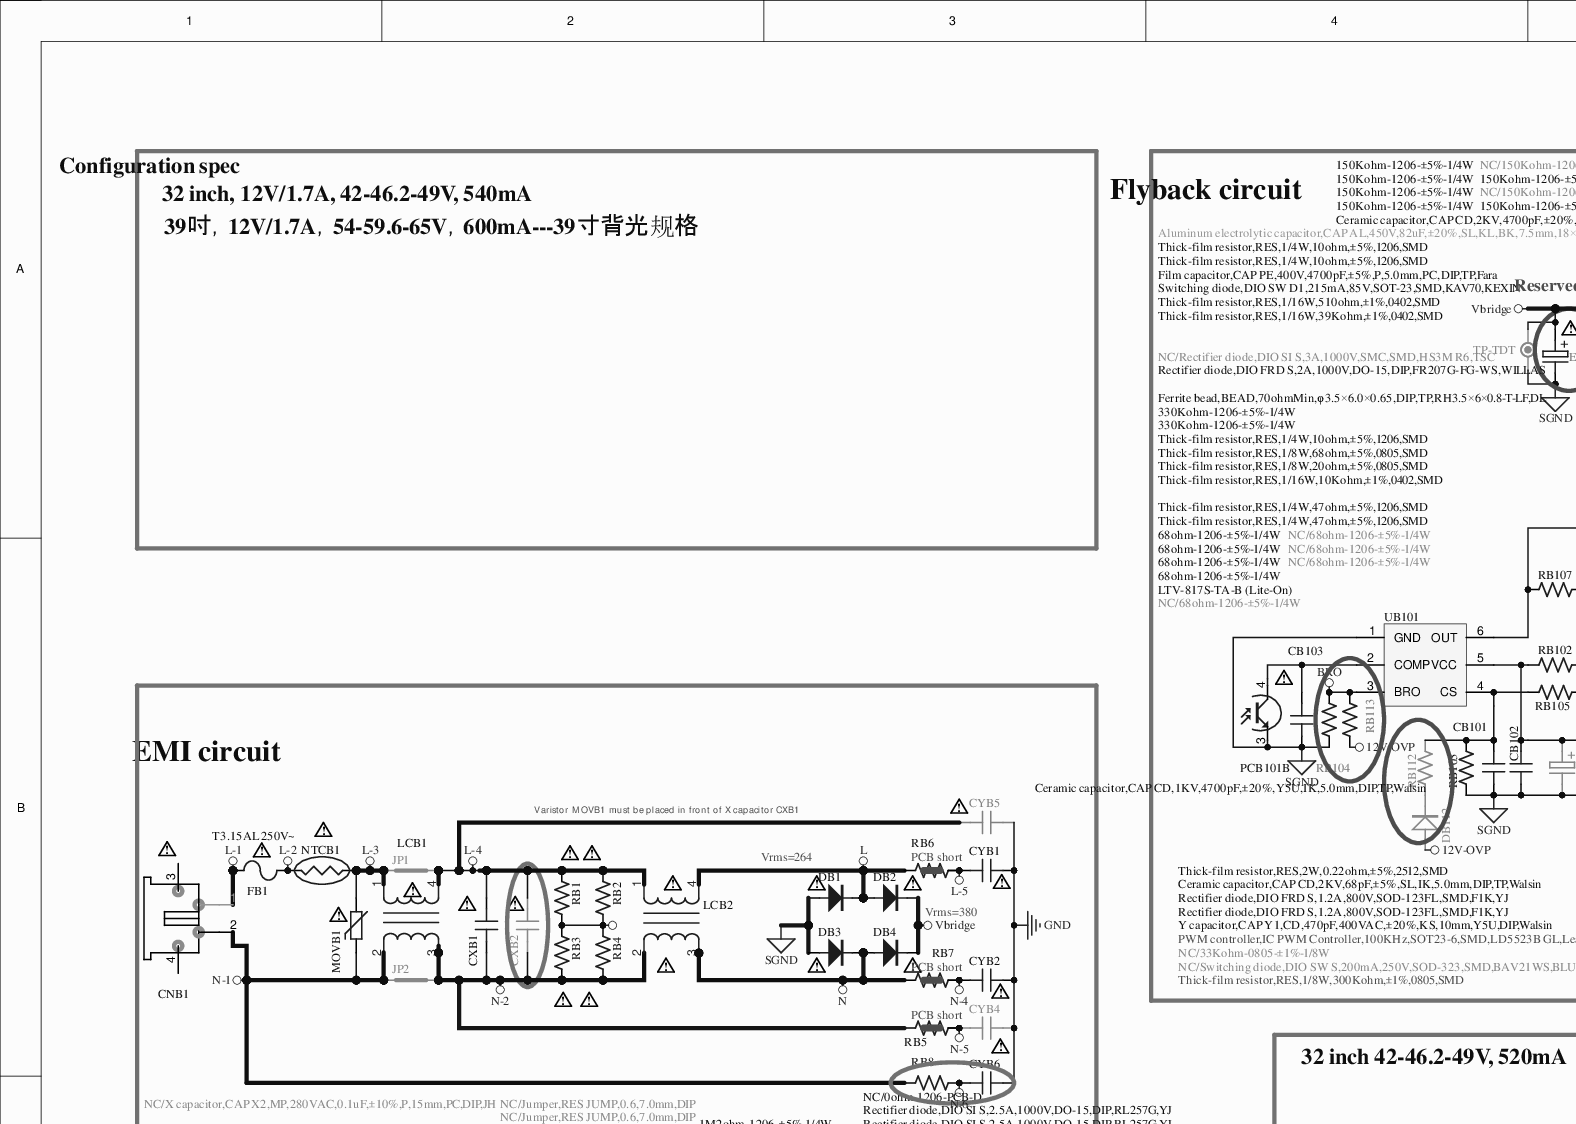
[diagram p0: MISC84438-4.SchDoc, top left]
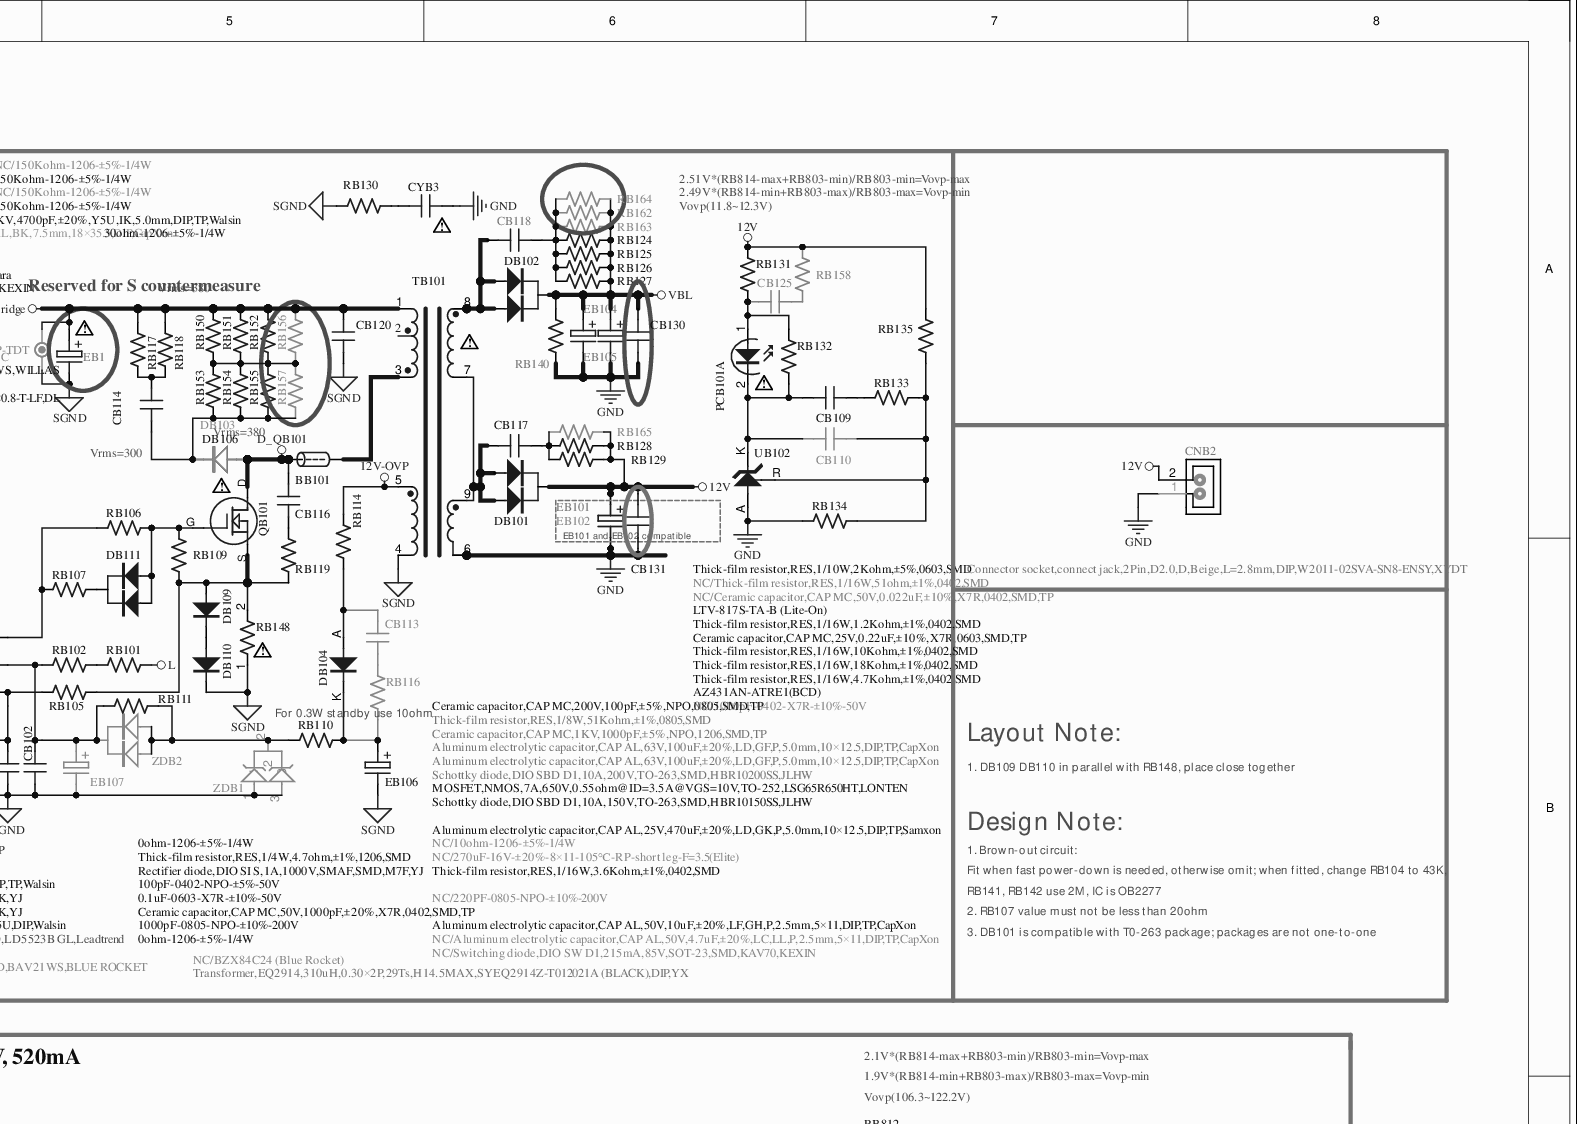
[diagram p1: MISC84438-4.SchDoc, top right]
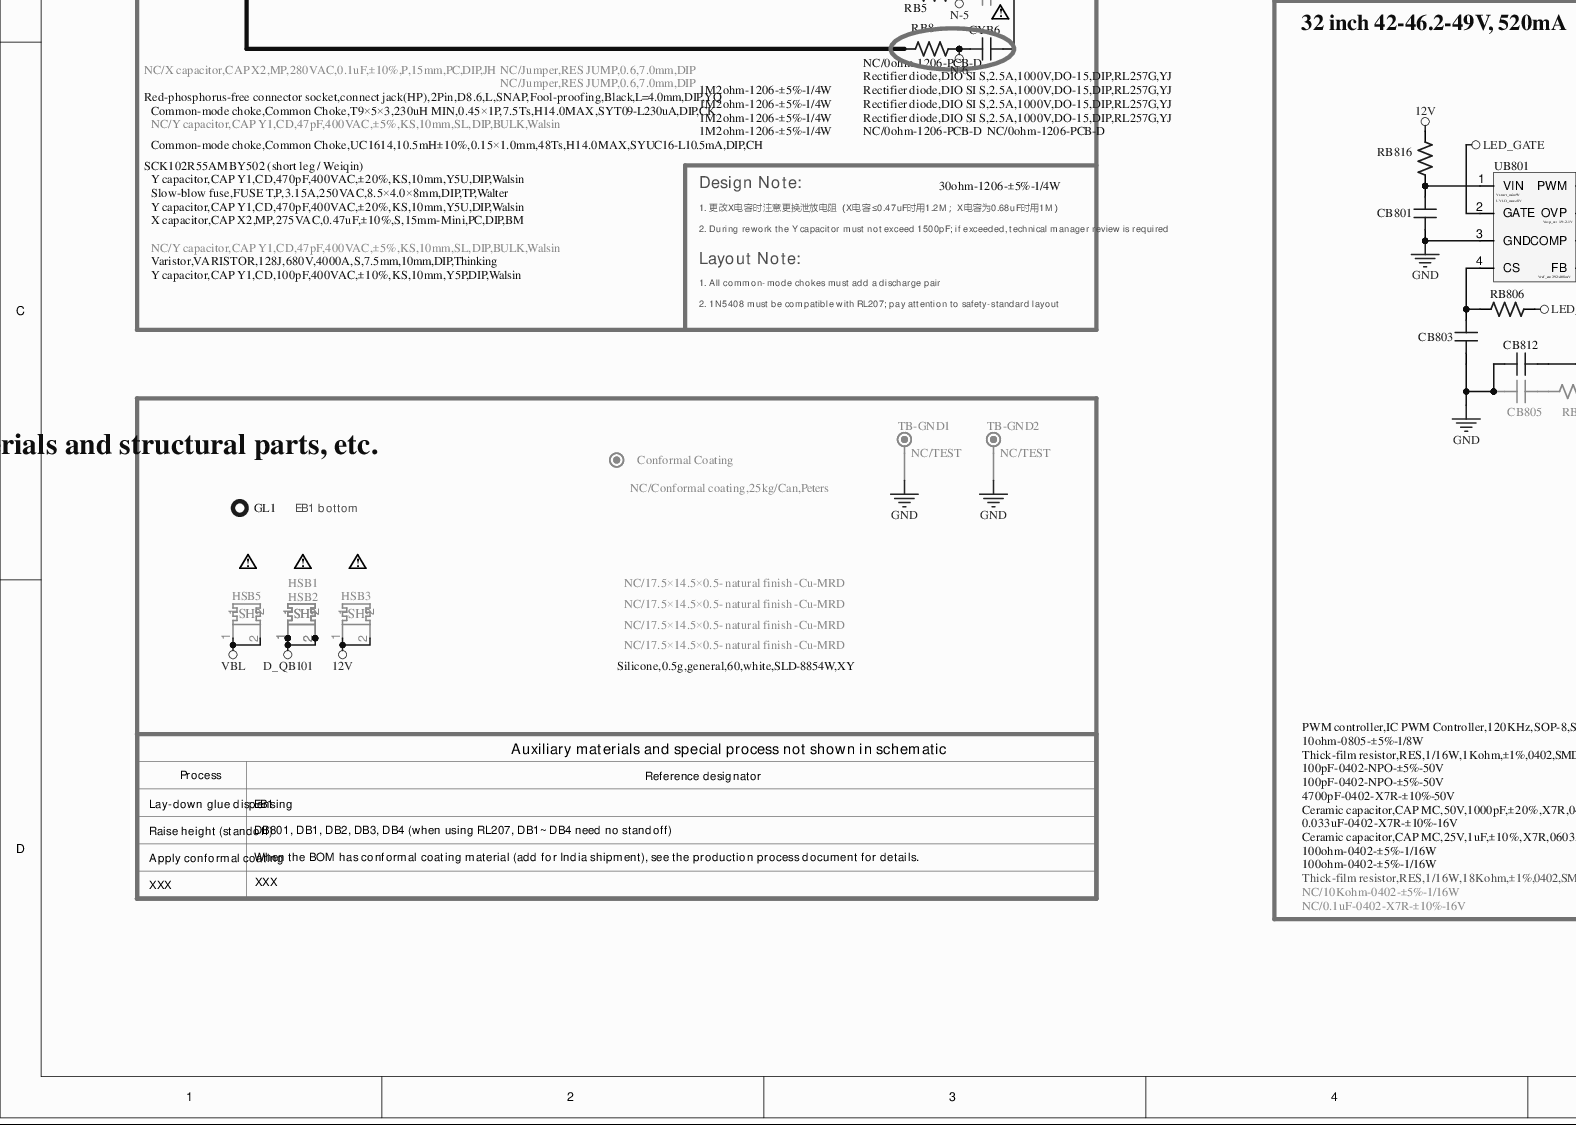
[diagram p2: MISC84438-4.SchDoc, bottom left]
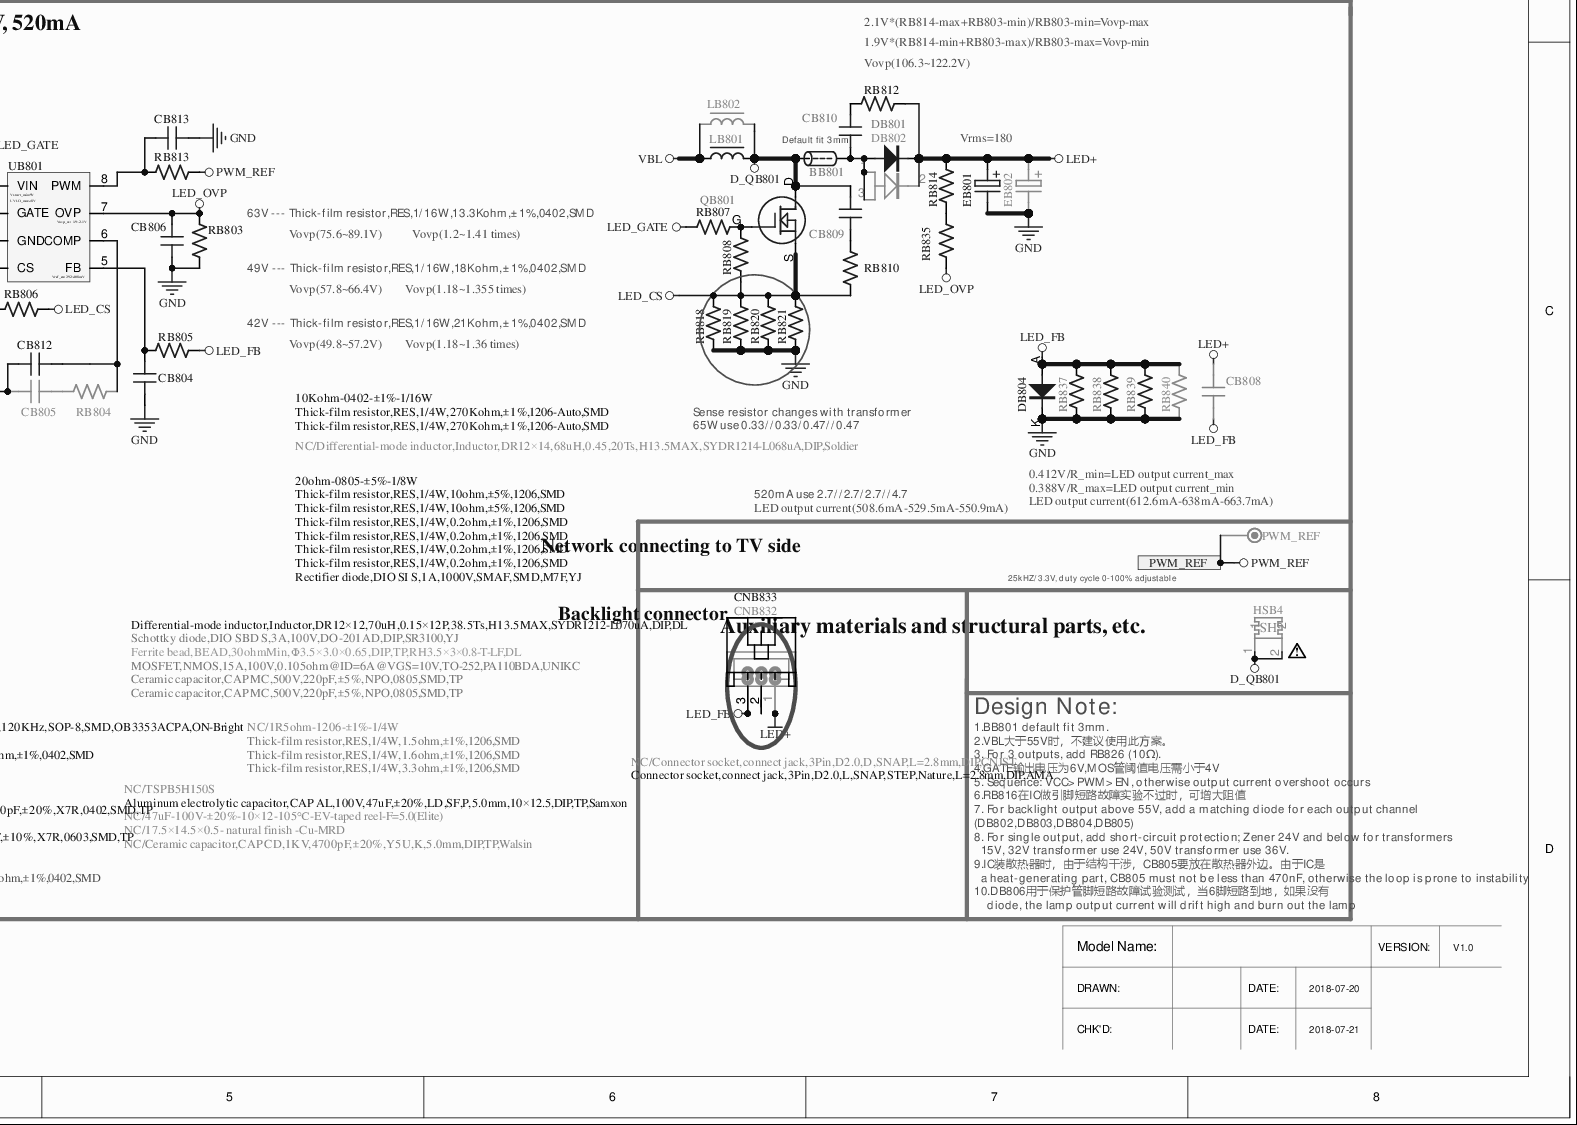
[diagram p3: MISC84438-4.SchDoc, bottom right]
# Altium project MISC84438-18.PrjPCB (part 7 of 8)

## Sheet MISC84438-4.SchDoc: MISC84438
size A2

### Parts
BB101  Ferrite bead,BEAD,70ohmMin,φ3.5×6.0×0.65,DIP,TP,RH3.5×6×0.8-T-LF,DL  [LB/3.5*6*12.5]
BB801  Ferrite bead,BEAD,30ohmMin,Φ3.5×3.0×0.65,DIP,TP,RH3.5×3×0.8-T-LF,DL  [LB/3.5*6*12.5]
CB101  100pF-0402-NPO-±5%-50V  [C0402]
CB102  0.1uF-0603-X7R-±10%-50V  [C0603]
CB103  Ceramic capacitor,CAP MC,50V,1000pF,±20%,X7R,0402,SMD,TP  [C0402]
CB109  Ceramic capacitor,CAP MC,25V,0.22uF,±10%,X7R,0603,SMD,TP  [C0603]
CB110  NC/1000pF-0402-X7R-±10%-50V  [C0402]
CB113  NC/220PF-0805-NPO-±10%-200V  [C0805]
CB114  Film capacitor,CAP PE,400V,4700pF,±5%,P,5.0mm,PC,DIP,TP,Fara  [CAP8*2.5-V-5]
CB116  Ceramic capacitor,CAP CD,2KV,68pF,±5%,SL,IK,5.0mm,DIP,TP,Walsin  [CAP6.5*5-V-5-1]
CB117  1000pF-0805-NPO-±10%-200V  [C0805]
CB118  Ceramic capacitor,CAP MC,1KV,1000pF,±5%,NPO,1206,SMD,TP  [C1206]
CB120  Ceramic capacitor,CAP CD,2KV,4700pF,±20%,Y5U,IK,5.0mm,DIP,TP,Walsin  [CAP10*4.5-V-5]
CB125  NC/Ceramic capacitor,CAP MC,50V,0.022uF,±10%,X7R,0402,SMD,TP  [C0402]
CB130  Ceramic capacitor,CAP CD,1KV,4700pF,±20%,Y5U,IK,5.0mm,DIP,TP,Walsin  [CAP10*4.5-V-5]
CB131  Ceramic capacitor,CAP MC,200V,100pF,±5%,NPO,0805,SMD,TP  [C0805]
CB801  Ceramic capacitor,CAP MC,25V,1uF,±10%,X7R,0603,SMD,TP  [C0603]
CB803  100pF-0402-NPO-±5%-50V  [C0402]
CB804  4700pF-0402-X7R-±10%-50V  [C0402]
CB805  NC/0.1uF-0402-X7R-±10%-16V  [C0402]
CB806  Ceramic capacitor,CAP MC,50V,1000pF,±20%,X7R,0402,SMD,TP  [C0402]
CB808  NC/Ceramic capacitor,CAP CD,1KV,4700pF,±20%,Y5U,K,5.0mm,DIP,TP,Walsin  [CAP10*4.5-V-5]
CB809  Ceramic capacitor,CAP MC,500V,220pF,±5%,NPO,0805,SMD,TP  [C0805]
CB810  Ceramic capacitor,CAP MC,500V,220pF,±5%,NPO,0805,SMD,TP  [C0805]
CB812  0.033uF-0402-X7R-±10%-16V  [C0402]
CB813  100pF-0402-NPO-±5%-50V  [C0402]
CNB1  Red-phosphorus-free connector socket,connect jack(HP),2Pin,D8.6,L,SNAP,Fool-proofing,Black,L=4.0mm,DIP,YQ  [CON2-H8.6-1]
CNB2  Connector socket,connect jack,2Pin,D2.0,D,Beige,L=2.8mm,DIP,W2011-02SVA-SN8-ENSY,XYDT  [SIP2/2.0D-1]
CNB832  NC/Connector socket,connect jack,3Pin,D2.0,D,SNAP,L=2.8mm,DIP,CNJST  [SIP3/2.0D-CP]
CNB833  Connector socket,connect jack,3Pin,D2.0,L,SNAP,STEP,Nature,L=2.8mm,DIP,AMA  [SIP3H/2.0D-3]
Conformal_Coating  NC/Conformal coating,25kg/Can,Peters  [Conformal Coating]
CXB1  X capacitor,CAP X2,MP,275VAC,0.47uF,±10%,S,15mm-Mini,PC,DIP,BM  [CAP18*8.5-V-15]
CXB2  NC/X capacitor,CAP X2,MP,280VAC,0.1uF,±10%,P,15mm,PC,DIP,JH  [CAP18*5*11.5-V-15]
CYB1  Y capacitor,CAP Y1,CD,470pF,400VAC,±20%,KS,10mm,Y5U,DIP,Walsin  [CAP13*5-V-10-1]
CYB2  Y capacitor,CAP Y1,CD,470pF,400VAC,±20%,KS,10mm,Y5U,DIP,Walsin  [CAP13*5-V-10-1]
CYB3  Y capacitor,CAP Y1,CD,470pF,400VAC,±20%,KS,10mm,Y5U,DIP,Walsin  [CAP13*5-V-10-1]
CYB4  NC/Y capacitor,CAP Y1,CD,47pF,400VAC,±5%,KS,10mm,SL,DIP,BULK,Walsin  [CAP13*5-V-10-1]
CYB5  NC/Y capacitor,CAP Y1,CD,47pF,400VAC,±5%,KS,10mm,SL,DIP,BULK,Walsin  [CAP13*5-V-10-1]
CYB6  Y capacitor,CAP Y1,CD,100pF,400VAC,±10%,KS,10mm,Y5P,DIP,Walsin  [CAP13*5-V-10-1]
DB1  Rectifier diode,DIO SI S,2.5A,1000V,DO-15,DIP,RL257G,YJ  [D2-H-15]
DB2  Rectifier diode,DIO SI S,2.5A,1000V,DO-15,DIP,RL257G,YJ  [D2-H-15]
DB3  Rectifier diode,DIO SI S,2.5A,1000V,DO-15,DIP,RL257G,YJ  [D2-H-15]
DB4  Rectifier diode,DIO SI S,2.5A,1000V,DO-15,DIP,RL257G,YJ  [D2-H-15]
DB101  Schottky diode,DIO SBD D1,10A,150V,TO-263,SMD,HBR10150SS,JLHW  [D2PAK3]
DB102  Schottky diode,DIO SBD D1,10A,200V,TO-263,SMD,HBR10200SS,JLHW  [D2PAK3]
DB103  NC/Rectifier diode,DIO SI S,3A,1000V,SMC,SMD,HS3M R6,TSC  [DIODE-SMC]
DB104  Rectifier diode,DIO SI S,1A,1000V,SMAF,SMD,M7F,YJ  [DIODE-S-2]
DB106  Rectifier diode,DIO FRD S,2A,1000V,DO-15,DIP,FR207G-FG-WS,WILLAS  [D2-H-15]
DB109  Rectifier diode,DIO FRD S,1.2A,800V,SOD-123FL,SMD,F1K,YJ  [DIODE-S-14]
DB110  Rectifier diode,DIO FRD S,1.2A,800V,SOD-123FL,SMD,F1K,YJ  [DIODE-S-14]
DB111  Switching diode,DIO SW D1,215mA,85V,SOT-23,SMD,KAV70,KEXIN  [SO-23]
DB112  NC/Switching diode,DIO SW S,200mA,250V,SOD-323,SMD,BAV21WS,BLUE ROCKET  [DIODE-S-12]
DB801  Schottky diode,DIO SBD S,3A,100V,DO-201AD,DIP,SR3100,YJ  [D3-H-20-2]
DB802  NC/TSPB5H150S  [DIODE-S-13]
DB804  Rectifier diode,DIO SI S,1A,1000V,SMAF,SMD,M7F,YJ  [DIODE-S-2]
EB1  Aluminum electrolytic capacitor,CAP AL,450V,82uF,±20%,SL,KL,BK,7.5mm,18×35.5,DIP,CapXon  [EC(18*41)-H-7.5-1]
EB101  Aluminum electrolytic capacitor,CAP AL,25V,470uF,±20%,LD,GK,P,5.0mm,10×12.5,DIP,TP,Samxon  [EC(10*12.5)-V-5]
EB102  NC/270uF-16V-±20%-8×11-105℃-RP-short leg-F=3.5(Elite)  [EC(8*11)-V-3.5]
EB104  Aluminum electrolytic capacitor,CAP AL,63V,100uF,±20%,LD,GF,P,5.0mm,10×12.5,DIP,TP,CapXon  [EC(10*12.5)-V-5]
EB105  Aluminum electrolytic capacitor,CAP AL,63V,100uF,±20%,LD,GF,P,5.0mm,10×12.5,DIP,TP,CapXon  [EC(10*12.5)-V-5]
EB106  Aluminum electrolytic capacitor,CAP AL,50V,10uF,±20%,LF,GH,P,2.5mm,5×11,DIP,TP,CapXon  [EC(5*11)-V-2.5]
EB107  NC/Aluminum electrolytic capacitor,CAP AL,50V,4.7uF,±20%,LC,LL,P,2.5mm,5×11,DIP,TP,CapXon  [EC(5*11)-V-2.5]
EB801  Aluminum electrolytic capacitor,CAP AL,100V,47uF,±20%,LD,SF,P,5.0mm,10×12.5,DIP,TP,Samxon  [EC(10*12.5)-V-5]
EB802  NC/47uF-100V-±20%-10×12-105℃-EV-taped reel-F=5.0(Elite)  [EC(10*12.5)-V-5]
FB1  Slow-blow fuse,FUSE T,P,3.15A,250VAC,8.5×4.0×8mm,DIP,TP,Walter  [FUSE8.5*4-V-5(T3.15AL 250V~)]
GL1  Silicone,0.5g,general,60,white,SLD-8854W,XY  [Silica gel-20]
HSB1  NC/17.5×14.5×0.5- natural finish -Cu-MRD  [HS038]
HSB2  NC/17.5×14.5×0.5- natural finish -Cu-MRD  [HS038]
HSB3  NC/17.5×14.5×0.5- natural finish -Cu-MRD  [HS038]
HSB4  NC/17.5×14.5×0.5- natural finish -Cu-MRD  [HS038]
HSB5  NC/17.5×14.5×0.5- natural finish -Cu-MRD  [HS038]
JP1  NC/Jumper,RES JUMP,0.6,7.0mm,DIP  [JP7.0]
JP2  NC/Jumper,RES JUMP,0.6,7.0mm,DIP  [JP7.0]
LB801  Differential-mode inductor,Inductor,DR12×12,70uH,0.15×12P,38.5Ts,H13.5MAX,SYDR1212-L070uA,DIP,DL  [L/LC2/15*14.5-V7.5]
LB802  NC/Differential-mode inductor,Inductor,DR12×14,68uH,0.45,20Ts,H13.5MAX,SYDR1214-L068uA,DIP,Soldier  [L(13.5*15.5)-V-5]
LCB1  Common-mode choke,Common Choke,T9×5×3,230uH MIN,0.45×1P,7.5Ts,H14.0MAX,SYT09-L230uA,DIP,CK  [L/LC4/12.8*10-V-6*7]
LCB2  Common-mode choke,Common Choke,UC1614,10.5mH±10%,0.15×1.0mm,48Ts,H14.0MAX,SYUC16-L10.5mA,DIP,CH  [L/LC4/21*17-H-17*13]
MOVB1  Varistor,VARISTOR,128J,680V,4000A,S,7.5mm,10mm,DIP,Thinking  [VR(13*5)-V-7.5]
NTCB1  SCK102R55AMBY502 (short leg / Weiqin)  [NTC(10*5)-V5]
PCB101  LTV-817S-TA-B (Lite-On)  [OC4-S-1]  (parts A,B of 2)
PWM_REF  NC/TEST  [TP_BL]  (value not drawn)
QB101  MOSFET,NMOS,7A,650V,0.55ohm@ID=3.5A@VGS=10V,TO-252,LSG65R650HT,LONTEN  [D2PAK3]
QB801  MOSFET,NMOS,15A,100V,0.105ohm@ID=6A@VGS=10V,TO-252,PA110BDA,UNIKC  [TO-252-GDS]
RB1  1M2ohm-1206-±5%-1/4W  [R1206]
RB2  1M2ohm-1206-±5%-1/4W  [R1206]
RB3  1M2ohm-1206-±5%-1/4W  [R1206]
RB4  1M2ohm-1206-±5%-1/4W  [R1206]
RB5  NC/0ohm-1206-PCB-D  [R1206SC]
RB6  NC/0ohm-1206-PCB-D  [R1206SC]
RB7  NC/0ohm-1206-PCB-D  [R1206SC]
RB8  30ohm-1206-±5%-1/4W  [R1206]
RB101  330Kohm-1206-±5%-1/4W  [R1206]
RB102  330Kohm-1206-±5%-1/4W  [R1206]
RB103  Thick-film resistor,RES,1/16W,3.6Kohm,±1%,0402,SMD  [R0402]
RB104  Thick-film resistor,RES,1/16W,39Kohm,±1%,0402,SMD  [R0402]
RB105  Thick-film resistor,RES,1/16W,510ohm,±1%,0402,SMD  [R0402]
RB106  Thick-film resistor,RES,1/8W,68ohm,±5%,0805,SMD  [R0805]
RB107  Thick-film resistor,RES,1/8W,20ohm,±5%,0805,SMD  [R0805]
RB109  Thick-film resistor,RES,1/16W,10Kohm,±1%,0402,SMD  [R0402]
RB110  0ohm-1206-±5%-1/4W  [R1206]
RB111  0ohm-1206-±5%-1/4W  [R1206]
RB112  NC/33Kohm-0805-±1%-1/8W  [R0805]
RB113  Thick-film resistor,RES,1/8W,300Kohm,±1%,0805,SMD  [R0805]
RB114  Thick-film resistor,RES,1/4W,4.7ohm,±1%,1206,SMD  [R1206]
RB116  NC/10ohm-1206-±5%-1/4W  [R1206]
RB117  Thick-film resistor,RES,1/4W,10ohm,±5%,1206,SMD  [R1206]
RB118  Thick-film resistor,RES,1/4W,10ohm,±5%,1206,SMD  [R1206]
RB119  Thick-film resistor,RES,1/4W,10ohm,±5%,1206,SMD  [R1206]
RB124  68ohm-1206-±5%-1/4W  [R1206]
RB125  68ohm-1206-±5%-1/4W  [R1206]
RB126  68ohm-1206-±5%-1/4W  [R1206]
RB127  68ohm-1206-±5%-1/4W  [R1206]
RB128  Thick-film resistor,RES,1/4W,47ohm,±5%,1206,SMD  [R1206]
RB129  Thick-film resistor,RES,1/4W,47ohm,±5%,1206,SMD  [R1206]
RB130  30ohm-1206-±5%-1/4W  [R1206]
RB131  Thick-film resistor,RES,1/10W,2Kohm,±5%,0603,SMD  [R0603]
RB132  Thick-film resistor,RES,1/16W,1.2Kohm,±1%,0402,SMD  [R0402]
RB133  Thick-film resistor,RES,1/16W,10Kohm,±1%,0402,SMD  [R0402]
RB134  Thick-film resistor,RES,1/16W,4.7Kohm,±1%,0402,SMD  [R0402]
RB135  Thick-film resistor,RES,1/16W,18Kohm,±1%,0402,SMD  [R0402]
RB140  Thick-film resistor,RES,1/8W,51Kohm,±1%,0805,SMD  [R0805]
RB148  Thick-film resistor,RES,2W,0.22ohm,±5%,2512,SMD  [R2512-1]
RB150  150Kohm-1206-±5%-1/4W  [R1206]
RB151  150Kohm-1206-±5%-1/4W  [R1206]
RB152  150Kohm-1206-±5%-1/4W  [R1206]
RB153  150Kohm-1206-±5%-1/4W  [R1206]
RB154  150Kohm-1206-±5%-1/4W  [R1206]
RB155  150Kohm-1206-±5%-1/4W  [R1206]
RB156  NC/150Kohm-1206-±5%-1/4W  [R1206]
RB157  NC/150Kohm-1206-±5%-1/4W  [R1206]
RB158  NC/Thick-film resistor,RES,1/16W,51ohm,±1%,0402,SMD  [R0402]
RB162  NC/68ohm-1206-±5%-1/4W  [R1206]
RB163  NC/68ohm-1206-±5%-1/4W  [R1206]
RB164  NC/68ohm-1206-±5%-1/4W  [R1206]
RB165  NC/68ohm-1206-±5%-1/4W  [R1206]
RB803  Thick-film resistor,RES,1/16W,18Kohm,±1%,0402,SMD  [R0402]
RB804  NC/10Kohm-0402-±5%-1/16W  [R0402]
RB805  100ohm-0402-±5%-1/16W  [R0402]
RB806  Thick-film resistor,RES,1/16W,1Kohm,±1%,0402,SMD  [R0402]
RB807  20ohm-0805-±5%-1/8W  [R0805]
RB808  10Kohm-0402-±1%-1/16W  [R0402]
RB810  Thick-film resistor,RES,1/4W,10ohm,±5%,1206,SMD  [R1206]
RB812  Thick-film resistor,RES,1/4W,10ohm,±5%,1206,SMD  [R1206]
RB813  100ohm-0402-±5%-1/16W  [R0402]
RB814  Thick-film resistor,RES,1/4W,270Kohm,±1%,1206-Auto,SMD  [R1206]
RB816  10ohm-0805-±5%-1/8W  [R0805]
RB818  Thick-film resistor,RES,1/4W,0.2ohm,±1%,1206,SMD  [R1206]
RB819  Thick-film resistor,RES,1/4W,0.2ohm,±1%,1206,SMD  [R1206]
RB820  Thick-film resistor,RES,1/4W,0.2ohm,±1%,1206,SMD  [R1206]
RB821  Thick-film resistor,RES,1/4W,0.2ohm,±1%,1206,SMD  [R1206]
RB835  Thick-film resistor,RES,1/4W,270Kohm,±1%,1206-Auto,SMD  [R1206]
RB837  Thick-film resistor,RES,1/4W,1.5ohm,±1%,1206,SMD  [R1206]
RB838  Thick-film resistor,RES,1/4W,1.6ohm,±1%,1206,SMD  [R1206]
RB839  Thick-film resistor,RES,1/4W,3.3ohm,±1%,1206,SMD  [R1206]
RB840  NC/1R5ohm-1206-±1%-1/4W  [R1206]
TB101  Transformer,EQ2914,310uH,0.30×2P,29Ts,H14.5MAX,SYEQ2914Z-T012021A (BLACK),DIP,YX  [T/EQ2914*9-1]
TB-GND1  NC/TEST  [TP-10]
TB-GND2  NC/TEST  [TP-10]
TP-TDT  NC/  [TP-TDT]  (value not drawn)
UB101  PWM controller,IC PWM Controller,100KHz,SOT23-6,SMD,LD5523B GL,Leadtrend  [SOT-26]
UB102  AZ431AN-ATRE1(BCD)  [SOT-23-RAK]
UB801  PWM controller,IC PWM Controller,120KHz,SOP-8,SMD,OB3353ACPA,ON-Bright  [SO-8A]
ZDB1  NC/BZX84C24 (Blue Rocket)  [SO-23]
ZDB2  NC/Switching diode,DIO SW D1,215mA,85V,SOT-23,SMD,KAV70,KEXIN  [SO-23]

### Blocks framed on the sheet
EB101 and EB102 compatible: CB131 EB101 EB102
EMI circuit: CNB1 CXB1 CXB2 CYB1 CYB2 CYB4-CYB6 DB1-DB4 FB1 JP1 JP2 LCB1 LCB2 MOVB1 NTCB1 RB1-RB8
Auxiliary materials and structural parts, etc.: Conformal_Coating GL1 HSB1-HSB3 HSB5 TB-GND1 TB-GND2

### Ports
PWM_REF

### Nets
12V: CB131.1 CNB2.2 DB101.2 EB101.1 EB102.1 HSB3.1 HSB3.2 RB128.2 RB129.2 RB131.2 RB135.1 RB158.2 RB165.2 RB816.1
12V-OVP: DB112.A RB113.2 RB114.2 TB101.5
BRO: RB104.2 RB113.1 UB101.3(BRO)
D_QB101: BB101.1 CB116.2 DB103.A DB106.A HSB1.1 HSB1.2 HSB2.1 HSB2.2 QB101.2(D)
D_QB801: BB801.1 CB809.2 HSB4.1 HSB4.2 LB801.2 LB802.2 QB801.D
GND: CB130.1 CB131.2 CB801.1 CB803.2 CB804.2 CB805.1 CB806.2 CB812.1 CB813.1 CNB2.1 CYB1.2 CYB2.2 CYB3.2 CYB4.2 CYB5.2 CYB6.2 DB804.K EB101.2 EB102.2 EB104.2 EB105.2 EB801.2 EB802.2 RB134.1 RB140.2 RB803.1 RB818.2 RB819.2 RB820.2 RB821.2 RB837.1 RB838.1 RB839.2 RB840.1 TB101.6 TB-GND1.1 TB-GND2.1 UB102.A UB801.3(GND)
L: DB1.K DB2.A LCB2.4 RB6.1 RB101.1
L-1: CNB1.1 FB1.1
L-2: FB1.2 NTCB1.2
L-3: JP1.2 LCB1.1 MOVB1.1 NTCB1.1
L-4: CXB1.1 CXB2.2 CYB5.1 JP1.1 LCB1.4 LCB2.1 RB1.1 RB2.1
L-5: CYB1.1 RB6.2 RB6.3
L-N: RB1.2 RB2.2 RB3.1 RB4.1
LED+: CB808.2 CNB832.1 CNB833.1 DB801.K DB802.2 EB801.1 EB802.1 RB812.2 RB814.1
LED_CS: QB801.S RB806.2 RB808.1 RB810.2 RB818.1 RB819.1 RB820.1 RB821.1
LED_FB: CB808.1 CNB832.3 CNB833.3 DB804.A RB805.2 RB837.2 RB838.2 RB839.1 RB840.2
LED_GATE: RB807.1 UB801.2(GATE)
LED_OVP: CB806.1 RB803.2 RB835.2 UB801.7(OVP)
N: DB3.K DB4.A LCB2.3 RB7.1
N-1: CNB1.2 JP2.2 LCB1.2 MOVB1.2 RB8.1
N-2: CXB1.2 CXB2.1 JP2.1 LCB1.3 LCB2.2 RB3.2 RB4.2 RB5.1
N-4: CYB2.1 RB7.2 RB7.3
N-5: CYB4.1 RB5.2 RB5.3
N-6: CYB6.1 RB8.2
PWM_REF: PWM_REF.1 RB813.2 ; port PWM_REF
SGND: CB101.2 CB102.2 CB103.2 CB120.1 DB1.A DB3.A DB110.K EB1.2 EB106.2 EB107.2 PCB101.3 RB103.1 RB104.1 RB130.1 RB148.1 TB101.4 TP-TDT.2 UB101.1(GND) ZDB1.1 ZDB1.3
VBL: CB130.2 DB102.2 EB104.1 EB105.1 HSB5.1 HSB5.2 LB801.1 LB802.1 RB124.2 RB125.2 RB126.2 RB127.2 RB140.1 RB162.2 RB163.2 RB164.2
Vbridge: CB120.2 DB2.K DB4.K EB1.1 RB117.2 RB118.2 RB150.2 RB151.2 RB152.2 RB156.2 TB101.1 TP-TDT.1
NetBB101_2: BB101.2 TB101.3
NetBB801_2: BB801.2 CB810.1 DB801.A DB802.1(Anode_1) DB802.3(Anode_2)
NetCB101_1: CB101.1 RB103.2 RB105.1 RB112.1 UB101.4(CS)
NetCB102_1: CB102.1 EB107.1 RB102.2 RB111.1 UB101.5(VCC) ZDB2.2
NetCB103_1: CB103.1 PCB101.4 UB101.2(COMP)
NetCB109_1: CB109.1 CB110.1 PCB101.2 RB132.1 UB102.K
NetCB109_2: CB109.2 RB133.2
NetCB110_2: CB110.2 RB133.1 RB134.2 RB135.2 UB102.R
NetCB113_1: CB113.1 DB104.A RB114.1
NetCB113_2: CB113.2 RB116.1
NetCB114_1: CB114.1 RB117.1 RB118.1
NetCB114_2: CB114.2 DB103.K DB106.K RB153.1 RB154.1 RB155.1 RB157.1
NetCB116_1: CB116.1 RB119.2
NetCB117_1: CB117.1 DB101.1 DB101.3 TB101.7 TB101.9
NetCB117_2: CB117.2 RB128.1 RB129.1 RB165.1
NetCB118_1: CB118.1 DB102.1 DB102.3 TB101.8
NetCB118_2: CB118.2 RB124.1 RB125.1 RB126.1 RB127.1 RB162.1 RB163.1 RB164.1
NetCB125_1: CB125.1 PCB101.1 RB131.1 RB132.2
NetCB125_2: CB125.2 RB158.1
NetCB801_2: CB801.2 RB816.2 UB801.1(VIN)
NetCB803_1: CB803.1 RB806.1 UB801.4(CS)
NetCB804_1: CB804.1 RB805.1 UB801.5(FB)
NetCB805_2: CB805.2 RB804.1
NetCB809_1: CB809.1 RB810.1
NetCB810_2: CB810.2 RB812.1
NetCB812_2: CB812.2 RB804.2 UB801.6(COMP)
NetCB813_2: CB813.2 RB813.1 UB801.8(PWM)
NetCNB832_2: CNB832.2 CNB833.2
NetCYB3_1: CYB3.1 RB130.2
NetDB104_K: DB104.K EB106.1 RB110.2 RB116.2
NetDB109_A: DB109.A QB101.3(S) RB105.2 RB109.1 RB119.1 RB148.2
NetDB109_K: DB109.K DB110.A
NetDB111_1: DB111.1 DB111.3 QB101.1(G) RB106.2 RB109.2
NetDB111_2: DB111.2 RB107.2
NetDB112_K: DB112.K RB112.2
NetQB801_G: QB801.G RB807.2 RB808.2
NetRB101_2: RB101.2 RB102.1
NetRB106_1: RB106.1 RB107.1 UB101.6(OUT)
NetRB110_1: RB110.1 RB111.2 ZDB1.2 ZDB2.1 ZDB2.3
NetRB150_1: RB150.1 RB151.1 RB152.1 RB153.2 RB154.2 RB155.2 RB156.1 RB157.2
NetRB814_2: RB814.2 RB835.1

Not connected (* = marked no-connect by the designer): CNB1 3* 4*

### Layout directives
net class HOT: 12V, 12V-OVP, BRO, D_QB101, D_QB801, GND, L, L-1, L-2, L-3, L-4, L-5, L-N, LED+, LED_CS, LED_FB, LED_GATE, LED_OVP, N, N-1, N-2, N-4, N-5, N-6, PWM_REF, SGND, VBL, Vbridge
net class POWER: 12V, 12V-OVP, BRO, D_QB101, D_QB801, GND, L, L-1, L-2, L-3, L-4, L-5, L-N, LED+, LED_CS, LED_FB, LED_GATE, LED_OVP, N, N-1, N-2, N-4, N-5, N-6, PWM_REF, SGND, VBL, Vbridge

### Notes on the sheet
- Configuration spec
- 2.51V*(RB814-max+RB803-min)/RB803-min=Vovp-max
- 32 inch, 12V/1.7A, 42-46.2-49V, 540mA
- 39吋，12V/1.7A，54-59.6-65V，600mA---39寸背光规格
- Flyback circuit
- (near CYB3) !
- 2.49V*(RB814-min+RB803-max)/RB803-max=Vovp-min
- Vovp(11.8~12.3V)
- Reserved for S countermeasure
- (near EB1) !
- Vrms=380
- (near TB101) !
- !
- (near CB114) Vrms=300
- (near QB101) !
- (near RB148) !
- (near RB116) For 0.3W standby use 10ohm
- Varistor MOVB1 must be placed in front of X capacitor CXB1
- (near CYB5) !
- 1. DB109 DB110 in parallel with RB148, place close together
- Layout Note:
- (near CNB1) !
- (near FB1) !
- (near NTCB1) !
- (near DB1) Vrms=264
- 1. Brown-out circuit:
- Fit when fast power-down is needed, otherwise omit; when fitted, change RB104 to 43K,
- Design Note:
- (near MOVB1) !
- (near LCB1) !
- (near CXB1) !
- (near CXB2) !
- (near LCB2) !
- (near DB1) !
- (near DB2) Vrms=380
- (near CYB1) !
- RB141, RB142 use 2M, IC is OB2277
- 2. RB107 value must not be less than 20ohm
- 3. DB101 is compatible with T0-263 package; packages are not one-to-one
- (near RB3) !
- (near DB3) !
- (near CYB2) !
- (near CYB4) !
- 32 inch 42-46.2-49V, 520mA
- 2.1V*(RB814-max+RB803-min)/RB803-min=Vovp-max
- 1.9V*(RB814-min+RB803-max)/RB803-max=Vovp-min
- Vovp(106.3~122.2V)
- (near CB810) Default fit 3mm
- Vrms=180
- 1. 更改X电容时注意更换泄放电阻（X电容≤0.47uF时用1.2M；X电容为0.68uF时用1M）
- 2. During rework the Y capacitor must not exceed 1500pF; if exceeded, technical manager review is required
- 63V --- Thick-film resistor,RES,1/16W,13.3Kohm,±1%,0402,SMD
- Vovp(75.6~89.1V)
- Vovp(1.2~1.41 times)
- 1. All common-mode chokes must add a discharge pair
- 2. 1N5408 must be compatible with RL207; pay attention to safety-standard layout
- 49V --- Thick-film resistor,RES,1/16W,18Kohm,±1%,0402,SMD
- 42V --- Thick-film resistor,RES,1/16W,21Kohm,±1%,0402,SMD
- Vovp(57.8~66.4V)
- Vovp(1.18~1.355 times)
- Vovp(49.8~57.2V)
- Vovp(1.18~1.36 times)
- Sense resistor changes with transformer
- 65W use 0.33//0.33/0.47//0.47
- EB1 bottom
- 520mA use 2.7//2.7/2.7//4.7
- LED output current(508.6mA-529.5mA-550.9mA)
- 0.412V/R_min=LED output current_max
- (near PWM_REF) 0.388V/R_max=LED output current_min
- (near PWM_REF) LED output current(612.6mA-638mA-663.7mA)
- Network connecting to TV side
- 25kHZ/3.3V, duty cycle 0-100% adjustable
- Backlight connector
- Auxiliary materials and structural parts, etc.
- (near HSB4) !
- 1.BB801 default fit 3mm.
- Process
- Auxiliary materials and special process not shown in schematic
- Reference designator
- 6.RB816在IC做引脚短路故障实验不过时，可增大阻值
- 3. For 3 outputs, add RB826 (10Ω).
- 2.VBL大于55V时，不建议使用此方案。
- 4.GATE输出电压为6V,MOS管阈值电压需小于4V
- 5. Sequence: VCC>PWM>EN, otherwise output current overshoot occurs
- Lay-down glue dispensing
- Raise height (standoff)
- Apply conformal coating
- EB1
- DB801, DB1, DB2, DB3, DB4 (when using RL207, DB1~DB4 need no standoff)
- When the BOM has conformal coating material (add for India shipment), see the production process document for details.
- 8. For single output, add short-circuit protection; Zener 24V and below for transformers
- 7. For backlight output above 55V, add a matching diode for each output channel
- (DB802,DB803,DB804,DB805)
- 9.IC装散热器时，由于结构干涉，CB805要放在散热器外边。由于IC是
- 15V, 32V transformer use 24V, 50V transformer use 36V.
- XXX
- 10.DB806用于保护管脚短路故障试验测试，当6脚短路到地，如果没有
- a heat-generating part, CB805 must not be less than 470nF, otherwise the loop is prone to instability
- diode, the lamp output current will drift high and burn out the lamp
- Model Name:
- DRAWN:
- XXXXXXXXXXXXXXXXX
- PERSON_A
- DATE:
- 2018-07-20
- VERSION:
- V1.0
- CHK'D:
- PERSON_B
- 2018-07-21
- Title
- Size:
- Date:
- A4
- Number:
- Time:
- Revision:
- Sheet
- of
- File:

### Library data of the parts
BB101 = φ3.5×6.0×0.65mm-CP(编带/秀益达)-DAI: Through-hole ferrite bead
BB801 = φ3.5×6.0×0.65mm-CP(编带/秀益达)-DLAI: Through-hole ferrite bead
CB101 CB803 CB813 = 100pF-0402-NPO-±5%-50V-D
CB102 CB109 = 0.1uF-0603-X7R-±10%-50V-D: CAP
CB103 = 1000pF-0402-X7R-±10%-50V-D
CB110 CB125 CB806 = 1000pF-0402-X7R-±10%-50V-D: CAP
CB113 CB131 = 220PF-0805-NPO-±10%-200V-D: CAP
CB114 = C242G472J20A201(编带/法拉)-DAI: CAP
CB116 = 004.003.0001889-DHAI: Ceramic capacitor,CAP CD,1KV,100pF,±5%,SL,OK,5.0mm,DIP,TP,TDK-DHAI
CB117 = 1000pF-0805-NPO-±10%-200V-D: CAP
CB118 = 陶瓷电容,CAP MC,1KV,4700pF,±10%,X7R,1206,SMD,TP,ISND-D
CB120 CB130 CB808 = 004.003.0001665: Ceramic capacitor,CAP CD,1KV,4700pF,±20%,Y5U,K,5.0mm,DIP,TP,Walsin-DHAI
CB801 = 1uf-0603-X7R-±10%-25V-D
CB804 = 4700pF-0402-X7R-±10%-50V-D
CB805 = 0.1uF-0402-X7R-±10%-16V-D
CB809 CB810 = 004.003.0001392: Ceramic capacitor,CAP MC,500V,47pF,±5%,NPO,0805,SMD,TP,WALSIN-D
CB812 = 0.033uF-0402-X7R-±10%-16V-D
CNB1 = 连接插座,connect jack,2Pin,D8.6,L,SNAP,Fool-proofing,Black,L=4.0mm,DIP,YQ-DLMI: AC socket, side exit (figure-eight)
CNB2 = XXX.XXX.0001753: Connector socket,connect jack,2Pin,D2.0,D,L=2.8mm,DIP,AMA-DHMI
CNB832 = XXX.XXX.0001754: Connector socket,connect jack,3Pin,D2.0,D,L=2.8mm,DIP,AMA-DHMI
CNB833 = 3PIN-2.0-L-H-G-带扣-带台阶-J-DLMI
Conformal_Coating = 三防漆,25kg/Can,Peters
CXB1 = X电容,CAP X2,MP,275VAC,0.47uF,±10%,S,15mm-Mini,PC,DIP,BM-DHMI: CAP
CXB2 = PX104K3ID19H200D9R(凯励)-DHMI: X capacitor
CYB1-CYB6 = Y电容,CAP Y1,CD,470pF,400VAC,±20%,KS,10mm,Y5U,DIP,Walsin-DHMI: Y1 capacitor
DB1-DB4 DB106 = RL207G(编带/GOOD-ARK)-DLAI: Diode
DB101 = 004.005.0000140-D: Rectifier diode,DIO SI D1,10A,150V,TO-263,SMD,MBRB10150CT,GOOD-ARK-D
DB102 = 004.005.0000473: Rectifier diode,DIO FRD D1,10A,400V,TO-263,SMD,MURB1040S,GOOD-ARK-D
DB103 = 整流二极管,DIO SI S,3A,1000V,SMC,SMD,HS3M R6,TSC-D: Diode
DB104 DB804 = M7(WEJ)-D: Diode
DB109 DB110 = 整流二极管,DIO FRD S,1.2A,800V,eSGA,SMD,R12K,GOOD-ARK-D
DB111 ZDB2 = LBAV70LT1G(LRC)-D: Diode
DB112 = BAV21WS-D: Diode
DB801 = 肖特基二极管,DIO SBD S,3A,150V,DO-201AD,DIP,SR315 A0G,TSC-DLMI: Diode
DB802 = TSPB5H150S-D: Diode
EB1 = 100uF-450V-±20%-18×41-105℃-KS-折脚开槽(CapXon)-S对策-DLMI: Electrolytic
EB101 = 470uF-25V-±20%-10×12.5-105℃-GF-编带-F=5.0(CapXon)-DHAI: Electrolytic
EB102 = 270uF-16V-±20%-8×11-105℃-RP-短脚-F=3.5(Elite)-DHMI: CAP
EB104 EB105 = 100uF-63V-±20%-10×12.5-105℃-GF-编带-F=5.0(CapXon)-DHAI: Electrolytic
EB106 EB107 = 10uF-50V-±20%-5×11-105℃-GH-编带-F=2.5(CapXon)-DHAI: Electrolytic
EB801 EB802 = 47uF-100V-±20%-10×12-105℃-EV-编带-F=5.0(Elite)-DHAI: Electrolytic
FB1 = 004.026.0000010-DHMI: Slow-blow fuse,FUSE T,P,3.15A,250VAC,8.5×4.0×8mm,DIP,TP,Walter-DHMI
GL1 = 005.002.0000011: Silicone,0.2g,general,60,white,SLD-8854W,XY-DHMI
HSB1-HSB5 = 17.5×14.5×0.5-本色-Cu-MRD-D: Heatsink
JP1 JP2 = 004.002.0002101-DLAI: Jumper,RES JUMP,0.6,7.0mm,DIP-DLAI
LB801 = SYDR1212-L003-EDL-DHMI: I-type inductor
LB802 = 差模电感,Inductor,DR12×14,68uH,0.45,20Ts,H13.5MAX,SYDR1214-L068uA,DIP,Soldier-DHMI: I-type inductor
LCB1 = 004.004.0002338-DHMI: Common-mode choke,Common Choke,T9×5×3,230uH MIN,0.45×1P,7.5Ts,H14.0MAX,SYT09-L230uA,DIP,CK-DHMI
LCB2 = 004.004.0002597-DHMI: Common-mode choke,Common Choke,UC1614,10.5mH±10%,0.15×1.0mm,48Ts,H14.0MAX,SYUC16-L10.5mA,DIP,CH-DHMI
MOVB1 = TVR10561KSW(为勤)-DHMI: Varistor
NTCB1 = SCK102R55AMBY502(短脚/为勤)-DHMI: Thermistor
PCB101 = LTV-817S-TA-B(光宝)-DMI: Optocoupler
PWM_REF TB-GND1 TB-GND2 TP-TDT = TEST
QB101 = 004.007.0000227-D: MOSFET,NMOS,13.7A,650V,0.22ohm@ID=6.9A@VGS=10V,D2PAK,TK14G65W,TOSHIBA-D
QB801 = AOD4454(AOS)-D: N Channel Single MOSFET
RB1-RB4 = 1M2ohm-1206-±5%-1/4W-D: RES
RB5-RB7 = 0ohm-1206-PCB-D
RB8 RB110 RB111 RB116-RB119 RB130 RB810 RB812 = 10ohm-1206-±5%-1/4W-D: RES
RB101 RB102 = 330Kohm-1206-±5%-1/4W-D: RES
RB103 = 6K8ohm-0402-±1%-1/16W-D
RB104 = 27Kohm-0402-±1%-1/16W-D
RB105 = 510ohm-0402-±1%-1/16W-D
RB106 = 68ohm-0805-±5%-1/8W-D
RB107 RB807 = 20ohm-0805-±5%-1/8W-D: RES
RB109 RB133 RB808 = 10Kohm-0402-±1%-1/16W-D
RB112 RB113 RB140 = 51Kohm-0805-±1%-1/8W-D: RES
RB114 = 4R7ohm-1206-±1%-1/4W-D: RES
RB124-RB127 RB162-RB165 = 68ohm-1206-±5%-1/4W-D: RES
RB128 RB129 = 47ohm-1206-±5%-1/4W-D: RES
RB131 = 2Kohm-0603-±5%-1/10W-D
RB132 RB806 = 1Kohm-0402-±1%-1/16W-D
RB134 = 4K7ohm-0402-±1%-1/16W-D: RES
RB135 = 18Kohm-0402-±1%-1/16W-D: RES
RB148 = 004.002.0001050: Thick-film resistor,RES,2W,0.22ohm,±5%,2512,SMD-D
RB150-RB157 = 100Kohm-1206-±5%-1/4W-D: RES
RB158 = 3Kohm-0402-±1%-1/16W-D
RB803 = 9K1ohm-0402-±1%-1/16W-D
RB804 = 10Kohm-0402-±5%-1/16W-D
RB805 = 100ohm-0402-±5%-1/16W-D: RES
RB813 = 100ohm-0402-±1%-1/16W-D
RB814 RB835 = 004.002.0001261: Thick-film resistor,RES,1/4W,510Kohm,±1%,1206-Auto,SMD-D
RB816 = 33ohm-0805-±5%-1/8W-D
RB818-RB821 = 0R3ohm-1206-±5%-1/4W-D
RB837 RB838 = 1R5ohm-1206-±1%-1/4W-D: RES
RB839 = 2R2ohm-1206-±1%-1/4W-D: RES
RB840 = 1R6ohm-1206-±1%-1/4W-D: RES
TB101 = 004.004.0002082: Transformer,EQ2914,270uH,0.35×2P,25Ts,H14.5MAX,SYEQ2914Z-T012021A (BLACK),DIP,YX-DHMI
UB101 = LD7537RGL(通嘉)-D: IC
UB102 = AZ431AN-ATRE1(BCD)-D: SMD 431 (shunt regulator)
UB801 = OB3350CPA(OB)-D: IC
ZDB1 = LBZX84C24LT1G(LRC)-D: Diode